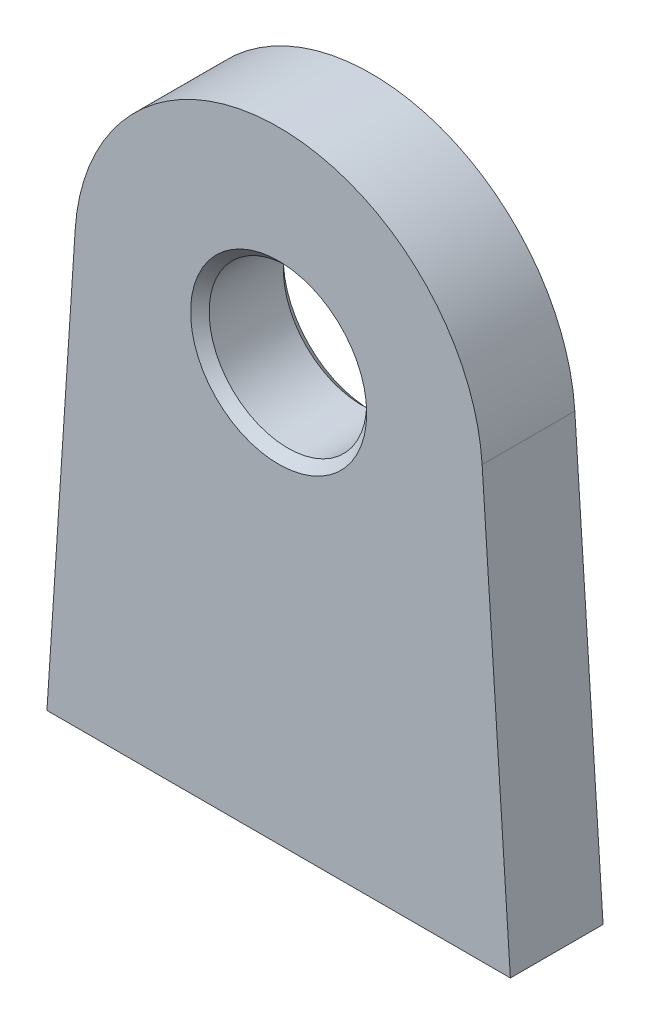
SolidWorks part; units mm, degrees
material "Q235B"
ref_plane "Front Plane" through (0, 0, 0) normal (0, 0, 1) x (1, 0, 0)
ref_plane "Top Plane" through (0, 0, 0) normal (0, 1, 0) x (1, 0, 0)
ref_plane "Right Plane" through (0, 0, 0) normal (1, 0, 0) x (0, 0, -1)
other "Configuration Table"
sketch "Sketch1" plane through (0, 0, 0) normal (0, 0, 1) x (1, 0, 0)
  line L0 (0, 0) -> (50, 0)
  line L1 (50, 0) -> (46.9528, 46.4404)
  line L2 (0, 0) -> (3.0472, 46.4404)
  arc A0 (46.9528, 46.4404) -> (3.0472, 46.4404) centre (25, 45) ccw
  circle A1 centre (25, 45) radius 8.5
  dimension "D4" = 44
  dimension "D1" = 50
  dimension "D2" = 25
  dimension "D3" = 45
extrude "Boss-Extrude1" add sketch "Sketch1" along normal blind 10
chamfer "Chamfer1" distance 1 angle 45 2 edges at (33.5, 45, 0) (33.5, 45, 10)
